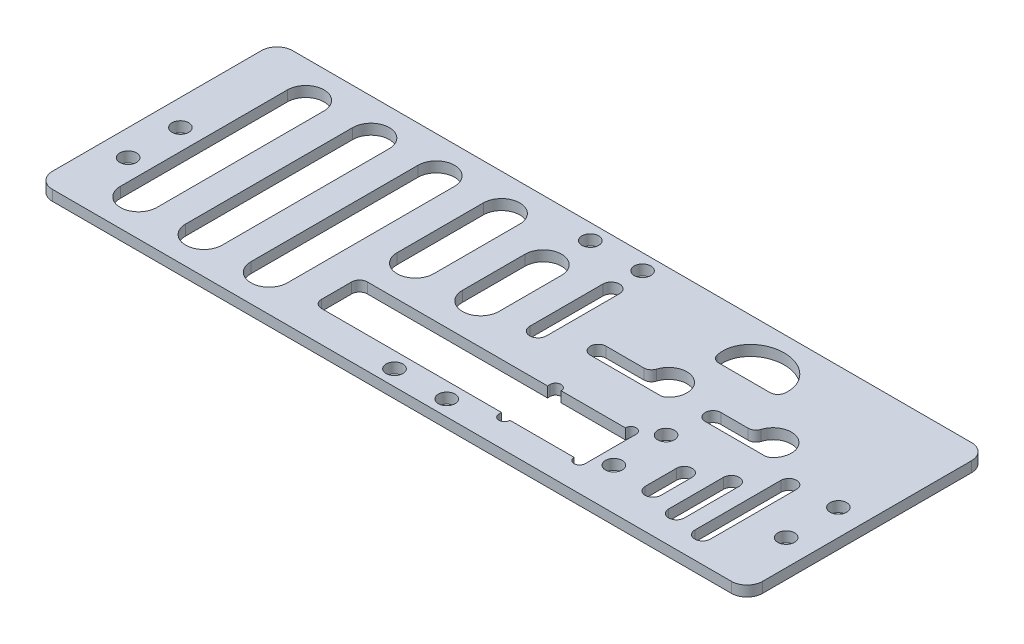
SolidWorks part; units mm, degrees
material "Thornel Mat VMA"
ref_plane "Front Plane" through (0, 0, 0) normal (0, 0, 1) x (1, 0, 0)
ref_plane "Top Plane" through (0, 0, 0) normal (0, 1, 0) x (1, 0, 0)
ref_plane "Right Plane" through (0, 0, 0) normal (1, 0, 0) x (0, 0, -1)
sketch "Sketch1" plane through (0, 0, 0) normal (0, 1, 0) x (1, 0, 0)
  line L0 (0, 23) -> (0, -23) construction
  line L1 (68, -23) -> (-68, -23)
  line L2 (68, -23) -> (68, 23)
  line L3 (68, 23) -> (-68, 23)
  line L4 (-68, -23) -> (-68, 23)
  line L5 (68, -23) -> (-68, 23) construction
  line L6 (68, 23) -> (-68, -23) construction
  line L7 (-63, -0.5) -> (-63, -10.5) construction
  line L8 (-2.5, -20) -> (7.5, -20) construction
  line L9 (34.5, -5) -> (34.5, -15) construction
  line L10 (63, -0.5) -> (63, -10.5) construction
  line L11 (-68, 0) -> (68, 0) construction
  line L12 (5, 20) -> (-5, 20) construction
  circle A0 centre (-63, -0.5) radius 1.6
  circle A1 centre (-63, -10.5) radius 1.6
  circle A2 centre (-2.5, -20) radius 1.6
  circle A3 centre (7.5, -20) radius 1.6
  circle A6 centre (63, -10.5) radius 1.6
  circle A7 centre (63, -0.5) radius 1.6
  circle A8 centre (5, 20) radius 1.6
  circle A9 centre (-5, 20) radius 1.6
  circle A12 centre (34.5, -5) radius 1.6
  circle A13 centre (34.5, -15) radius 1.6
  point P0 (0, 0)
  dimension "D2" = 12.5
  dimension "D4" = 3.2
  dimension "D11" = 33.5
  dimension "D1" = 136
  dimension "D3" = 10
  dimension "D5" = 5
  dimension "D6" = 3
  dimension "D7" = 46
  dimension "D8" = 3
  dimension "D10" = 65.5
  dimension "D12" = 8
extrude "Boss-Extrude1" add sketch "Sketch1" along normal blind 2
sketch "Sketch2" plane through (0, 2, 0) normal (0, 1, 0) x (1, 0, 0)
  line L0 (-68, -23) -> (68, -23) construction
  line L1 (-55.5, 16) -> (-55.5, -16) construction
  line L2 (-52, 16) -> (-52, -16)
  line L3 (17.1, -7.7) -> (29.4, -7.7)
  line L4 (-59, 16) -> (-59, -16)
  line L5 (-68, 0) -> (68, 0) construction
  line L6 (-21, -8.2) -> (-21, -17)
  line L9 (17.1, -17.5) -> (29.4, -17.5)
  line L12 (31.5, -7.7) -> (31.5, -17.5)
  line L15 (-21, -17) -> (15, -17)
  line L18 (15, -17) -> (15, -17.5)
  line L21 (15, -7.7) -> (15, -8.2)
  line L24 (15, -8.2) -> (-21, -8.2)
  line L25 (-68, 23) -> (-68, -23) construction
  line L26 (68, -23) -> (68, 23) construction
  line L27 (-43, 16) -> (-43, -16) construction
  line L28 (-39.5, 16) -> (-39.5, -16)
  line L29 (-46.5, 16) -> (-46.5, -16)
  line L30 (-30.5, 16) -> (-30.5, -16) construction
  line L31 (-27, 16) -> (-27, -16)
  line L32 (-34, 16) -> (-34, -16)
  line L36 (-5.5, 11.5) -> (-5.5, -0.5) construction
  line L37 (-2, 11.5) -> (-2, -0.5)
  line L38 (-9, 11.5) -> (-9, -0.5)
  line L39 (0, 23) -> (0, -23) construction
  line L40 (68, 23) -> (-68, 23) construction
  line L41 (42.5, 4) -> (36, 4)
  line L50 (36, 1) -> (47.8028, 1)
  line L53 (42.5, -15.5) -> (42.5, -9.5) construction
  line L54 (41, -15.5) -> (41, -9.5)
  line L55 (44, -15.5) -> (44, -9.5)
  line L56 (48.5, -17) -> (48.5, -6.5) construction
  line L57 (47, -17) -> (47, -6.5)
  line L58 (50, -17) -> (50, -6.5)
  line L59 (54.5, -18) -> (54.5, -1.5) construction
  line L60 (53, -18) -> (53, -1.5)
  line L61 (56, -18) -> (56, -1.5)
  line L73 (22.5, 4) -> (14, 4)
  line L82 (27.8028, 1) -> (14, 1)
  line L100 (38.5554, 12) -> (26.5554, 12)
  line L107 (31.4548, 8.5039) -> (33.4517, 19.8292) construction
  line L108 (5, 0) -> (5, 14) construction
  line L109 (3.4, 0) -> (3.4, 14)
  line L110 (6.6, 0) -> (6.6, 14)
  line L111 (26.052, 15.2952) -> (38.8545, 13.0378) construction
  line L112 (-18, -0.5) -> (-18, 16) construction
  line L113 (-21.5, -0.5) -> (-21.5, 16)
  line L114 (-14.5, -0.5) -> (-14.5, 16)
  circle A18 centre (34.5, -15) radius 1.6 construction
  arc A19 (31.5, -7.7) -> (29.4, -7.7) centre (30.45, -7.7) ccw
  arc A20 (29.4, -17.5) -> (31.5, -17.5) centre (30.45, -17.5) ccw
  arc A21 (17.1, -7.7) -> (15, -7.7) centre (16.05, -7.7) ccw
  arc A22 (15, -17.5) -> (17.1, -17.5) centre (16.05, -17.5) ccw
  arc A23 (-52, 16) -> (-59, 16) centre (-55.5, 16) ccw
  arc A24 (-59, -16) -> (-52, -16) centre (-55.5, -16) ccw
  arc A25 (-39.5, 16) -> (-46.5, 16) centre (-43, 16) ccw
  arc A26 (-46.5, -16) -> (-39.5, -16) centre (-43, -16) ccw
  arc A27 (-27, 16) -> (-34, 16) centre (-30.5, 16) ccw
  arc A28 (-34, -16) -> (-27, -16) centre (-30.5, -16) ccw
  arc A31 (-2, 11.5) -> (-9, 11.5) centre (-5.5, 11.5) ccw
  arc A32 (-9, -0.5) -> (-2, -0.5) centre (-5.5, -0.5) ccw
  circle A33 centre (-63, -10.5) radius 1.6 construction
  arc A42 (41, -15.5) -> (44, -15.5) centre (42.5, -15.5) ccw
  arc A43 (44, -9.5) -> (41, -9.5) centre (42.5, -9.5) ccw
  arc A44 (47, -17) -> (50, -17) centre (48.5, -17) ccw
  arc A45 (50, -6.5) -> (47, -6.5) centre (48.5, -6.5) ccw
  arc A46 (53, -18) -> (56, -18) centre (54.5, -18) ccw
  arc A47 (56, -1.5) -> (53, -1.5) centre (54.5, -1.5) ccw
  arc A84 (3.4, 0) -> (6.6, 0) centre (5, 0) ccw
  arc A85 (6.6, 14) -> (3.4, 14) centre (5, 14) ccw
  circle A86 centre (5, 20) radius 1.6 construction
  arc A87 (47.8028, 1) -> (42.5, 4) centre (46, 4) ccw
  arc A88 (36, 4) -> (36, 1) centre (36, 2.5) ccw
  arc A90 (14, 4) -> (14, 1) centre (14, 2.5) ccw
  arc A91 (27.8028, 1) -> (22.5, 4) centre (26, 4) ccw
  arc A92 (-21.5, -0.5) -> (-14.5, -0.5) centre (-18, -0.5) ccw
  arc A93 (-14.5, 16) -> (-21.5, 16) centre (-18, 16) ccw
  circle A94 centre (-5, 20) radius 1.6 construction
  ellipse E0 centre (32.4533, 14.1665) end of major axis (38.8545, 13.0378) minor radius 5.75 (38.5554, 12) -> (26.5554, 12) ccw
  point P21 (-55.5, 0)
  point P35 (-43, 0)
  point P42 (-30.5, 0)
  point P50 (-18, 7.75)
  point P56 (-5.5, 5.5)
  point P69 (5, 7)
  point P95 (42.5, -12.5)
  point P100 (48.5, -11.75)
  point P109 (54.5, -9.75)
  dimension "D1" = 5.5
  dimension "D4" = 1.05
  dimension "D6" = 0.5
  dimension "D9" = 3.5
  dimension "D15" = 4
  dimension "D16" = 1.5
  dimension "D26" = 3
  dimension "D39" = 12.5
  dimension "D40" = 8.5
  dimension "D49" = 6
  dimension "D27" = 3.5
  dimension "D29" = 12
  dimension "D31" = 22
  dimension "D33" = 11
  dimension "D2" = 9.8
  dimension "D5" = 16.5
  dimension "D7" = 0.5
  dimension "D8" = 36
  dimension "D10" = 32
  dimension "D3" = 3
  dimension "D11" = 3
  dimension "D12" = 12.5
  dimension "D13" = 12.5
  dimension "D14" = 12
  dimension "D17" = 3
  dimension "D18" = 3
  dimension "D19" = 1.5
  dimension "D20" = 1
  dimension "D21" = 5
  dimension "D22" = 3
  dimension "D23" = 6
  dimension "D24" = 8
  dimension "D25" = 5
  dimension "D28" = 10
  dimension "D30" = 10
  dimension "D32" = 22
  dimension "D34" = 12
  dimension "D35" = 35.5467
  dimension "D36" = 10
  dimension "D37" = 11.5
  dimension "D38" = 13
extrude "Cut-Extrude1" cut sketch "Sketch2" against normal through all
fillet "R1.5 cutout fillet" radius 1.5 8 edges at (-21, 1, 8.2) (-21, 1, 17) (38.5554, 1, -12) (26.5554, 1, -12) (22.5, 1, -4) (27.8028, 1, -1) (42.5, 1, -4) (47.8028, 1, -1)
fillet "R3 outer edge fillet" radius 3 4 edges at (-68, 1, -23) (68, 1, 23) (-68, 1, 23) (68, 1, -23)
